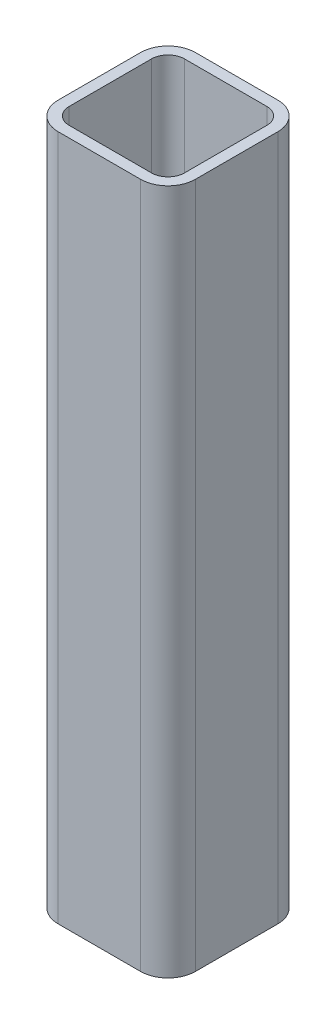
from build123d import *

# Parameters (mm, degrees)
BOSS_EXTRUDE1_DEPTH = 250


with BuildPart() as part:
    # Sketch1 → Boss-Extrude1 (new body)
    with BuildSketch(Plane(origin=(0, 0, 0), x_dir=(1, 0, 0), z_dir=(0, 1, 0))):
        with BuildLine():
            Line((-15, -25), (15, -25))
            ThreePointArc((15, -25), (22.071067812, -22.071067812), (25, -15))
            Line((25, -15), (25, 15))
            ThreePointArc((25, 15), (22.071067812, 22.071067812), (15, 25))
            Line((15, 25), (-15, 25))
            ThreePointArc((-15, 25), (-22.071067812, 22.071067812), (-25, 15))
            Line((-25, 15), (-25, -15))
            ThreePointArc((-25, -15), (-22.071067812, -22.071067812), (-15, -25))
        make_face()
        with BuildLine():
            Line((-15, 21), (15, 21))
            ThreePointArc((15, 21), (19.242640687, 19.242640687), (21, 15))
            Line((21, 15), (21, -15))
            ThreePointArc((21, -15), (19.242640687, -19.242640687), (15, -21))
            Line((15, -21), (-15, -21))
            ThreePointArc((-15, -21), (-19.242640687, -19.242640687), (-21, -15))
            Line((-21, -15), (-21, 15))
            ThreePointArc((-21, 15), (-19.242640687, 19.242640687), (-15, 21))
        make_face(mode=Mode.SUBTRACT)
    extrude(amount=BOSS_EXTRUDE1_DEPTH)


solid = part.part
